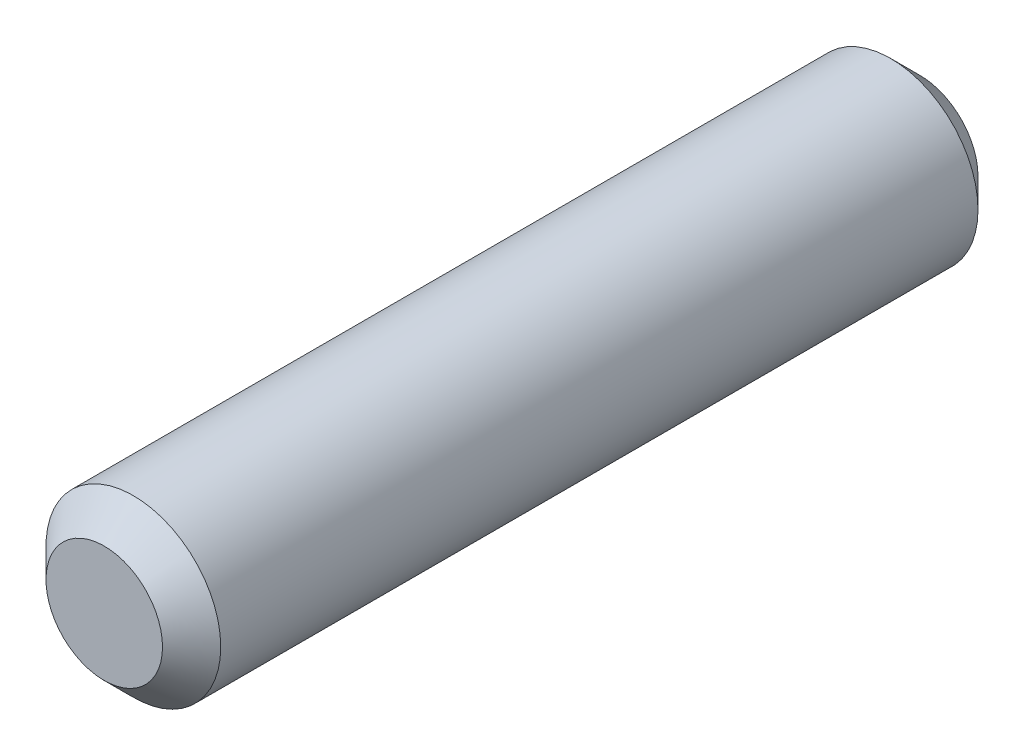
from build123d import *

# Parameters (mm, degrees)
SKETCH1_R           = 1.5
BOSS_EXTRUDE1_DEPTH = 14
CHAMFER1_SIZE       = 0.5


with BuildPart() as part:
    # Sketch1 → Boss-Extrude1 (new body)
    with BuildSketch(Plane.XY):
        Circle(SKETCH1_R)
    extrude(amount=BOSS_EXTRUDE1_DEPTH)

    # Chamfer1
    chamfer1_edges = [part.edges().sort_by_distance(p)[0] for p in [
        (-1.5, 0, 0),
        (-1.5, 0, 14),
    ]]
    chamfer(chamfer1_edges, length=CHAMFER1_SIZE)


solid = part.part
